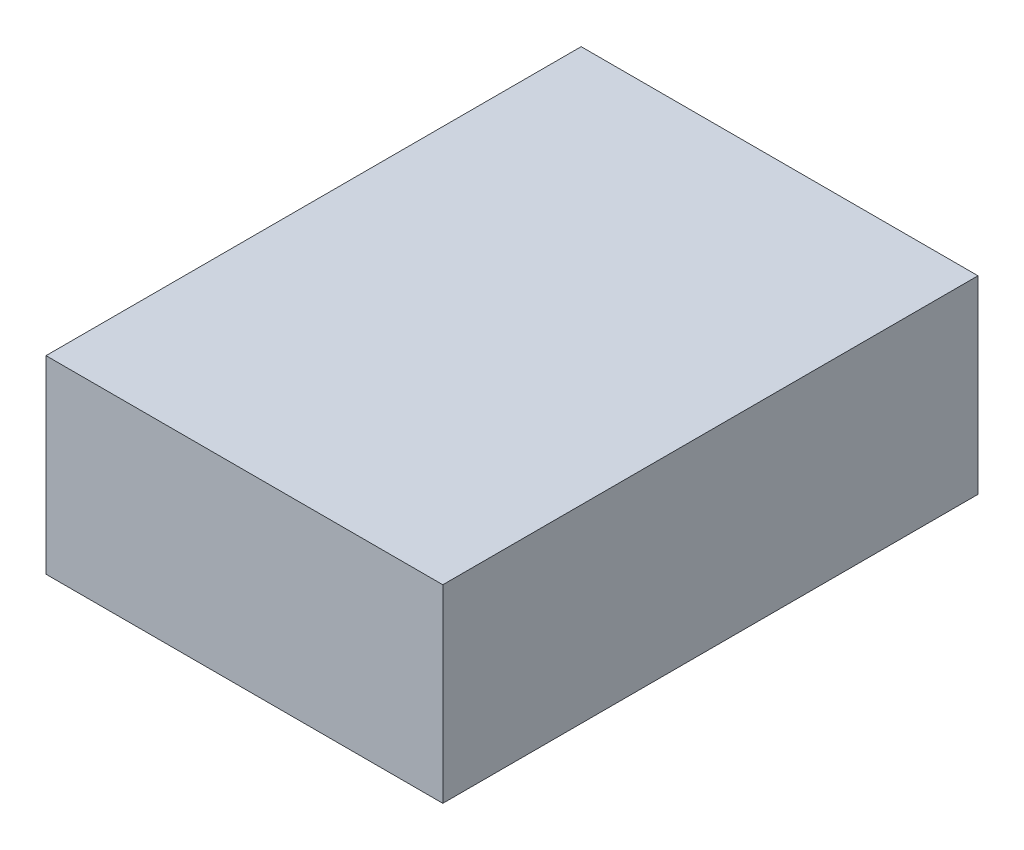
SolidWorks part; units mm, degrees
material "SPCC冷轧板喷塑"
ref_plane "前视基准面" through (0, 0, 0) normal (0, 0, 1) x (1, 0, 0)
ref_plane "上视基准面" through (0, 0, 0) normal (0, 1, 0) x (1, 0, 0)
ref_plane "右视基准面" through (0, 0, 0) normal (1, 0, 0) x (0, 0, -1)
other "Configuration Table"
sketch "草图1" plane through (0, 0, 0) normal (1, 0, 0) x (0, 0, -1)
  line L1 (367.5, -130) -> (-367.5, -130)
  line L2 (367.5, -130) -> (367.5, 130)
  line L3 (367.5, 130) -> (-367.5, 130)
  line L4 (-367.5, -130) -> (-367.5, 130)
  line L5 (367.5, -130) -> (-367.5, 130) construction
  line L6 (367.5, 130) -> (-367.5, -130) construction
  point P0 (0, 0)
  dimension "D1" = 735
  dimension "D2" = 260
extrude "凸台-拉伸1" add sketch "草图1" along normal mid plane 545
